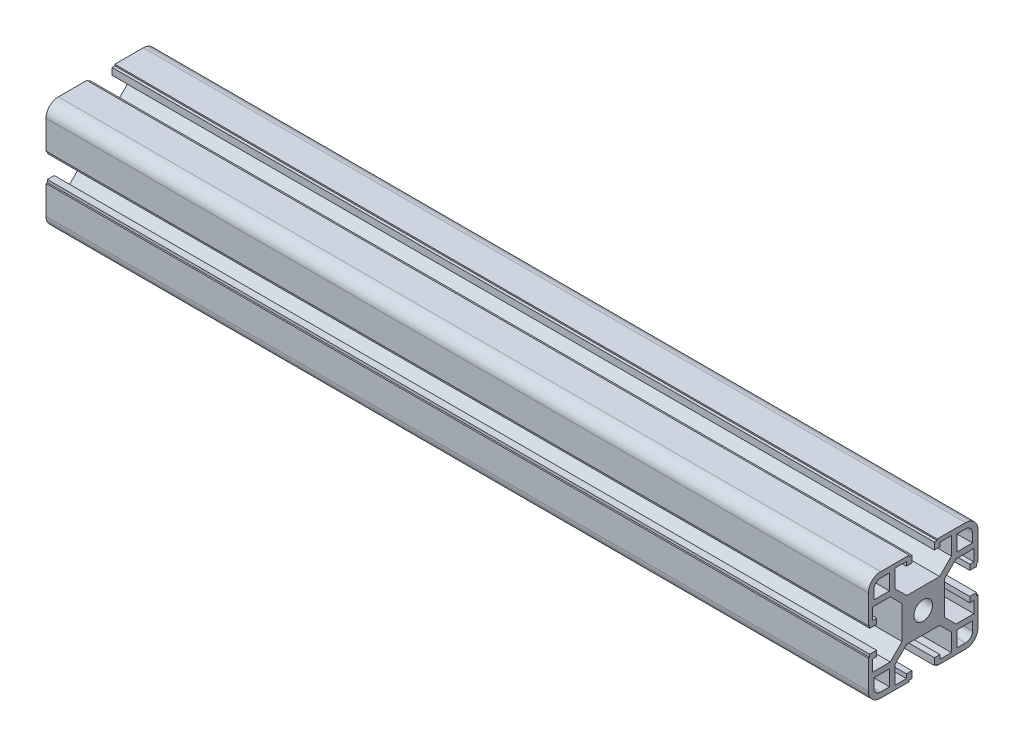
SolidWorks part; units mm, degrees
ref_plane "Front Plane" through (0, 0, 0) normal (0, 0, 1) x (1, 0, 0)
ref_plane "Top Plane" through (0, 0, 0) normal (0, 1, 0) x (1, 0, 0)
ref_plane "Right Plane" through (0, 0, 0) normal (1, 0, 0) x (0, 0, -1)
sketch "草图1" plane through (0, 0, 0) normal (0, 0, 1) x (1, 0, 0)
  line L0 (0, 0) -> (300, 0)
  dimension "D1" = 300
other "Aluminum profile 40 X 40B X R4.5(1)"
ref_plane "Plane1" through (0, 0, 0) normal (1, 0, 0) x (0, 1, 0)
sketch "Sketch1" plane through (0, 0, 0) normal (1, 0, 0) x (0, 1, 0)
  line L0 (-5.1, 20) -> (-5.1, 19.5)
  line L1 (-5.1, 19.5) -> (-4.1, 19.5)
  line L2 (-4.1, 19.5) -> (-4.1, 17)
  line L3 (-6.1, 18.5) -> (-10.3, 18.5)
  line L4 (-15.5, -20) -> (-5.1, -20)
  line L5 (-20, -15.5) -> (-20, -5.1)
  line L6 (15.5, 20) -> (5.1, 20)
  line L7 (20, 15.5) -> (20, 5.1)
  line L8 (0, 14.8756) -> (0, 0) construction
  line L9 (0, 0) -> (14.1675, 0) construction
  line L10 (-10.3, 18.5) -> (-10.3, 12)
  line L11 (-10.3, 12) -> (-6, 7.7)
  line L12 (-6, 7.7) -> (6, 7.7)
  line L13 (10.3, 12) -> (6, 7.7)
  line L14 (10.3, 18.5) -> (10.3, 12)
  line L15 (6.1, 18.5) -> (10.3, 18.5)
  line L16 (4.1, 19.5) -> (4.1, 17)
  line L17 (5.1, 19.5) -> (4.1, 19.5)
  line L18 (5.1, 20) -> (5.1, 19.5)
  line L19 (-5.1, 20) -> (-15.5, 20)
  line L20 (20, 5.1) -> (19.5, 5.1)
  line L21 (12.3, 18) -> (15.5, 18)
  line L22 (12.3, 18) -> (12.3, 12.3)
  line L23 (12.3, 12.3) -> (18, 12.3)
  line L24 (18, 15.5) -> (18, 12.3)
  line L25 (19.5, 5.1) -> (19.5, 4.1)
  line L26 (19.5, 4.1) -> (17, 4.1)
  line L27 (17, 6.1) -> (17, 4.1)
  line L28 (18.5, 6.1) -> (17, 6.1)
  line L29 (18.5, 6.1) -> (18.5, 10.3)
  line L30 (18.5, 10.3) -> (12, 10.3)
  line L31 (12, 10.3) -> (7.7, 6)
  line L32 (7.7, 6) -> (7.7, -6)
  line L33 (12, -10.3) -> (7.7, -6)
  line L34 (18.5, -10.3) -> (12, -10.3)
  line L35 (18.5, -6.1) -> (18.5, -10.3)
  line L36 (18.5, -6.1) -> (17, -6.1)
  line L37 (17, -4.1) -> (17, -6.1)
  line L38 (19.5, -4.1) -> (17, -4.1)
  line L39 (19.5, -5.1) -> (19.5, -4.1)
  line L40 (20, -5.1) -> (19.5, -5.1)
  line L41 (5.1, -20) -> (5.1, -19.5)
  line L42 (5.1, -19.5) -> (4.1, -19.5)
  line L43 (4.1, -19.5) -> (4.1, -17)
  line L44 (6.1, -17) -> (4.1, -17)
  line L45 (6.1, -18.5) -> (6.1, -17)
  line L46 (6.1, -18.5) -> (10.3, -18.5)
  line L47 (10.3, -18.5) -> (10.3, -12)
  line L48 (10.3, -12) -> (6, -7.7)
  line L49 (6, -7.7) -> (-6, -7.7)
  line L50 (-10.3, -12) -> (-6, -7.7)
  line L51 (-10.3, -18.5) -> (-10.3, -12)
  line L52 (-6.1, -18.5) -> (-10.3, -18.5)
  line L53 (-6.1, -18.5) -> (-6.1, -17)
  line L54 (-4.1, -17) -> (-6.1, -17)
  line L55 (-4.1, -19.5) -> (-4.1, -17)
  line L56 (-5.1, -19.5) -> (-4.1, -19.5)
  line L57 (-5.1, -20) -> (-5.1, -19.5)
  line L58 (-20, -5.1) -> (-19.5, -5.1)
  line L59 (5.1, -20) -> (15.5, -20)
  line L60 (-20, 5.1) -> (-20, 15.5)
  line L61 (-19.5, -5.1) -> (-19.5, -4.1)
  line L62 (-6.1, 18.5) -> (-6.1, 17)
  line L63 (-6.1, 17) -> (-4.1, 17)
  line L64 (6.1, 18.5) -> (6.1, 17)
  line L65 (4.1, 17) -> (6.1, 17)
  line L66 (-19.5, -4.1) -> (-17, -4.1)
  line L67 (-15.5, 18) -> (-12.3, 18)
  line L68 (-18, 15.5) -> (-18, 12.3)
  line L69 (-18, 12.3) -> (-12.3, 12.3)
  line L70 (-12.3, 18) -> (-12.3, 12.3)
  line L71 (-17, -6.1) -> (-17, -4.1)
  line L72 (-18.5, -6.1) -> (-17, -6.1)
  line L73 (-18.5, -6.1) -> (-18.5, -10.3)
  line L74 (-18.5, -10.3) -> (-12, -10.3)
  line L75 (-12, -10.3) -> (-7.7, -6)
  line L76 (-7.7, -6) -> (-7.7, 6)
  line L77 (-12, 10.3) -> (-7.7, 6)
  line L78 (-18.5, 10.3) -> (-12, 10.3)
  line L79 (-18.5, 6.1) -> (-18.5, 10.3)
  line L80 (-18.5, 6.1) -> (-17, 6.1)
  line L81 (-17, 4.1) -> (-17, 6.1)
  line L82 (-19.5, 4.1) -> (-17, 4.1)
  line L83 (-19.5, 5.1) -> (-19.5, 4.1)
  line L84 (-20, 5.1) -> (-19.5, 5.1)
  line L85 (20, -5.1) -> (20, -15.5)
  line L87 (-18, -12.3) -> (-12.3, -12.3)
  line L88 (-18, -12.3) -> (-18, -15.5)
  line L89 (-15.5, -18) -> (-12.3, -18)
  line L90 (-12.3, -12.3) -> (-12.3, -18)
  line L91 (12.3, -12.3) -> (18, -12.3)
  line L92 (12.3, -12.3) -> (12.3, -18)
  line L93 (12.3, -18) -> (15.5, -18)
  line L94 (18, -12.3) -> (18, -15.5)
  circle A0 centre (0, 0) radius 3.4
  arc A1 (-20, 15.5) -> (-15.5, 20) centre (-15.5, 15.5) cw
  arc A2 (20, 15.5) -> (15.5, 20) centre (15.5, 15.5) ccw
  arc A3 (-15.5, -20) -> (-20, -15.5) centre (-15.5, -15.5) cw
  arc A4 (15.5, -20) -> (20, -15.5) centre (15.5, -15.5) ccw
  arc A5 (-15.5, 18) -> (-18, 15.5) centre (-15.5, 15.5) ccw
  arc A6 (18, 15.5) -> (15.5, 18) centre (15.5, 15.5) ccw
  arc A7 (18, -15.5) -> (15.5, -18) centre (15.5, -15.5) cw
  arc A8 (-18, -15.5) -> (-15.5, -18) centre (-15.5, -15.5) ccw
  point P2 (0, 10)
  point P4 (0, 0)
  point P5 (-20, -20)
  point P6 (20, -20)
  point P7 (20, 20)
  point P8 (-20, 20)
  point P36 (-20, 20)
  point P39 (20, 20)
  point P121 (0, 0)
  dimension "D1" = 20.6
  dimension "D2" = 40
  dimension "D3" = 8.2
  dimension "D4" = 10.2
  dimension "D5" = 12.3
  dimension "D6" = 6.8
  dimension "D7" = 4.5
  dimension "D8" = 45
  dimension "D12" = 2
  dimension "D13" = 5.7
  dimension "D14" = 2
  dimension "D18" = 2.5
  dimension "D19" = 2.5
  dimension "D15" = 2.5
  dimension "D9" = 0.5
  dimension "D10" = 1.5
  dimension "D11" = 12
  dimension "D16" = 3
  dimension "D17" = 2
  dimension "D20" = 2
  dimension "D21" = 2
